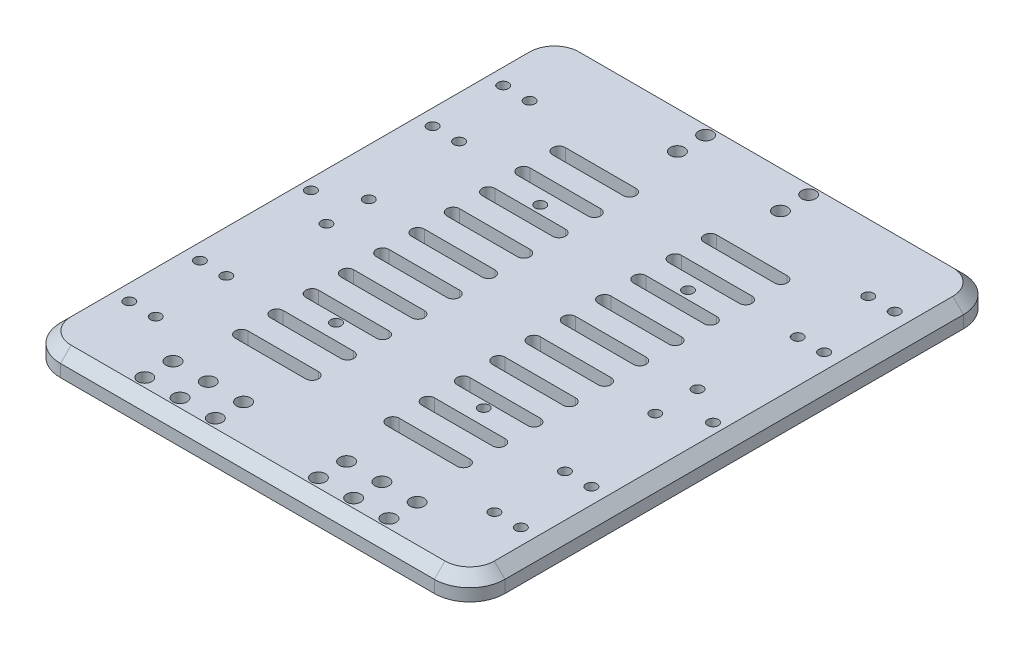
SolidWorks part; units mm, degrees
ref_plane "Front Plane" through (0, 0, 0) normal (0, 0, 1) x (1, 0, 0)
ref_plane "Top Plane" through (0, 0, 0) normal (0, 1, 0) x (1, 0, 0)
ref_plane "Right Plane" through (0, 0, 0) normal (1, 0, 0) x (0, 0, -1)
other "Configuration Table"
sketch "Sketch1" plane through (0, 0, 0) normal (0, 1, 0) x (1, 0, 0)
  line L1 (-63, -75) -> (63, -75)
  line L2 (-63, -75) -> (-63, 75)
  line L3 (-63, 75) -> (63, 75)
  line L4 (63, -75) -> (63, 75)
  line L5 (0, 75) -> (0, -75) construction
  line L6 (-63, 0) -> (63, 0) construction
  point P0 (0, 0)
  dimension "D1" = 126
  dimension "D2" = 150
extrude "Boss-Extrude1" add sketch "Sketch1" along normal blind 6.5
sketch "Sketch2" plane through (0, 6.5, 0) normal (0, 1, 0) x (1, 0, 0)
  line L0 (63, 75) -> (-63, 75) construction
  line L1 (-55.5, 33) -> (-48, 33) construction
  line L2 (-55.5, 33) -> (-55.5, 53) construction
  line L3 (-55.5, 53) -> (-48, 53) construction
  line L4 (-48, 33) -> (-48, 53) construction
  line L5 (-51.75, 53) -> (-51.75, 33) construction
  line L6 (-55.5, 43) -> (-48, 43) construction
  line L7 (-63, 75) -> (-63, -75) construction
  circle A0 centre (-55.5, 33) radius 1.5
  circle A1 centre (-48, 33) radius 1.5
  circle A2 centre (-48, 53) radius 1.5
  circle A3 centre (-55.5, 53) radius 1.5
  point P0 (-51.75, 43)
  dimension "D3" = 3
  dimension "D1" = 20
  dimension "D2" = 7.5
  dimension "D4" = 22
  dimension "D5" = 7.5
extrude "Cut-Extrude1" cut sketch "Sketch2" against normal blind 10
mirror "Mirror1" about plane through (0, 0, 0) normal (1, 0, 0) of "Cut-Extrude1"
mirror "Mirror2" about plane through (0, 0, 0) normal (0, 0, 1) of "Cut-Extrude1", "Mirror1"
fillet "Fillet1" radius 10 4 edges at (63, 3.25, 75) (-63, 3.25, 75) (63, 3.25, -75) (-63, 3.25, -75)
sketch "Sketch4" plane through (0, 6.5, 0) normal (0, 1, 0) x (1, 0, 0)
  line L0 (-63, 65) -> (-63, -65) construction
  line L1 (-57, 0) -> (-46.6077, -6) construction
  line L2 (-46.6077, -6) -> (-46.6077, 6) construction
  line L3 (-46.6077, 6) -> (-57, 0) construction
  circle A0 centre (-50.0718, 0) radius 3.4641 construction
  circle A1 centre (-46.6077, -6) radius 1.5
  circle A2 centre (-46.6077, 6) radius 1.5
  circle A3 centre (-57, 0) radius 1.5
  dimension "D3" = 3
  dimension "D1" = 12
  dimension "D2" = 6
extrude "Cut-Extrude3" cut sketch "Sketch4" against normal blind 10
mirror "Mirror3" about plane through (0, 0, 0) normal (1, 0, 0) of "Cut-Extrude3"
sketch "Sketch5" plane through (0, 6.5, 0) normal (0, 1, 0) x (1, 0, 0)
  line L0 (-53, -75) -> (53, -75) construction
  line L1 (63, -65) -> (63, 65) construction
  circle A0 centre (14.61, -61.5) radius 2
  circle A1 centre (14.61, -69.5) radius 2
  dimension "D1" = 4
  dimension "D2" = 13.5
  dimension "D3" = 48.39
  dimension "D4" = 8
extrude "Cut-Extrude4" cut sketch "Sketch5" against normal blind 20
mirror "Mirror4" about plane through (0, 0, 0) normal (1, 0, 0) of "Cut-Extrude4"
mirror "Mirror5" about plane through (0, 0, 0) normal (0, 0, 1) of "Cut-Extrude4", "Mirror4"
sketch "Sketch6" plane through (0, 6.5, 0) normal (0, 1, 0) x (1, 0, 0)
  circle A8 centre (14.61, -69.5) radius 2 construction
  circle A9 centre (14.61, -69.5) radius 2
  circle A10 centre (14.61, -61.5) radius 2 construction
  circle A11 centre (14.61, -61.5) radius 2
  circle A12 centre (24.61, -61.5) radius 2
  circle A13 centre (24.61, -69.5) radius 2
  circle A22 centre (34.61, -61.5) radius 2
  circle A23 centre (34.61, -69.5) radius 2
  circle A24 centre (-14.61, -61.5) radius 2 construction
  circle A25 centre (-14.61, -61.5) radius 2
  circle A26 centre (-14.61, -69.5) radius 2 construction
  circle A27 centre (-14.61, -69.5) radius 2
  circle A28 centre (-24.61, -61.5) radius 2
  circle A29 centre (-24.61, -69.5) radius 2
  circle A30 centre (-34.61, -61.5) radius 2
  circle A31 centre (-34.61, -69.5) radius 2
  dimension "D2" = 10
  dimension "D3" = 10
extrude "Cut-Extrude5" cut sketch "Sketch6" against normal through all
sketch "Sketch7" plane through (0, 6.5, 0) normal (0, 1, 0) x (1, 0, 0)
  line L0 (-31.4514, 44.7788) -> (-11.4514, 44.7788) construction
  line L1 (-31.4514, 46.5755) -> (-11.4514, 46.5755)
  line L2 (-31.4514, 42.9822) -> (-11.4514, 42.9822)
  line L3 (-31.4514, 34.7788) -> (-11.4514, 34.7788) construction
  line L4 (-31.4514, 36.5755) -> (-11.4514, 36.5755)
  line L5 (-31.4514, 32.9822) -> (-11.4514, 32.9822)
  line L6 (-31.4514, 24.7788) -> (-11.4514, 24.7788) construction
  line L7 (-31.4514, 26.5755) -> (-11.4514, 26.5755)
  line L8 (-31.4514, 22.9822) -> (-11.4514, 22.9822)
  line L9 (-31.4514, 14.7788) -> (-11.4514, 14.7788) construction
  line L10 (-31.4514, 16.5755) -> (-11.4514, 16.5755)
  line L11 (-31.4514, 12.9822) -> (-11.4514, 12.9822)
  line L12 (-31.4514, 4.7788) -> (-11.4514, 4.7788) construction
  line L13 (-31.4514, 6.5755) -> (-11.4514, 6.5755)
  line L14 (-31.4514, 2.9822) -> (-11.4514, 2.9822)
  line L15 (-31.4514, -5.2212) -> (-11.4514, -5.2212) construction
  line L16 (-31.4514, -3.4245) -> (-11.4514, -3.4245)
  line L17 (-31.4514, -7.0178) -> (-11.4514, -7.0178)
  line L18 (-31.4514, -15.2212) -> (-11.4514, -15.2212) construction
  line L19 (-31.4514, -13.4245) -> (-11.4514, -13.4245)
  line L20 (-31.4514, -17.0178) -> (-11.4514, -17.0178)
  line L21 (-31.4514, -25.2212) -> (-11.4514, -25.2212) construction
  line L22 (-31.4514, -23.4245) -> (-11.4514, -23.4245)
  line L23 (-31.4514, -27.0178) -> (-11.4514, -27.0178)
  line L24 (-31.4514, -35.2212) -> (-11.4514, -35.2212) construction
  line L25 (-31.4514, -33.4245) -> (-11.4514, -33.4245)
  line L26 (-31.4514, -37.0178) -> (-11.4514, -37.0178)
  line L27 (-31.4514, -45.2212) -> (-11.4514, -45.2212) construction
  line L28 (-31.4514, -43.4245) -> (-11.4514, -43.4245)
  line L29 (-31.4514, -47.0178) -> (-11.4514, -47.0178)
  line L30 (0, 0) -> (0, 32.0502) construction
  line L31 (31.4514, 44.7788) -> (11.4514, 44.7788) construction
  line L32 (31.4514, 46.5755) -> (11.4514, 46.5755)
  line L33 (31.4514, 42.9822) -> (11.4514, 42.9822)
  line L34 (31.4514, 34.7788) -> (11.4514, 34.7788) construction
  line L35 (31.4514, 36.5755) -> (11.4514, 36.5755)
  line L36 (31.4514, 32.9822) -> (11.4514, 32.9822)
  line L37 (31.4514, 24.7788) -> (11.4514, 24.7788) construction
  line L38 (31.4514, 26.5755) -> (11.4514, 26.5755)
  line L39 (31.4514, 22.9822) -> (11.4514, 22.9822)
  line L40 (31.4514, 14.7788) -> (11.4514, 14.7788) construction
  line L41 (31.4514, 16.5755) -> (11.4514, 16.5755)
  line L42 (31.4514, 12.9822) -> (11.4514, 12.9822)
  line L43 (31.4514, 4.7788) -> (11.4514, 4.7788) construction
  line L44 (31.4514, 6.5755) -> (11.4514, 6.5755)
  line L45 (31.4514, 2.9822) -> (11.4514, 2.9822)
  line L46 (31.4514, -5.2212) -> (11.4514, -5.2212) construction
  line L47 (31.4514, -3.4245) -> (11.4514, -3.4245)
  line L48 (31.4514, -7.0178) -> (11.4514, -7.0178)
  line L49 (31.4514, -15.2212) -> (11.4514, -15.2212) construction
  line L50 (31.4514, -13.4245) -> (11.4514, -13.4245)
  line L51 (31.4514, -17.0178) -> (11.4514, -17.0178)
  line L52 (31.4514, -25.2212) -> (11.4514, -25.2212) construction
  line L53 (31.4514, -23.4245) -> (11.4514, -23.4245)
  line L54 (31.4514, -27.0178) -> (11.4514, -27.0178)
  line L55 (31.4514, -35.2212) -> (11.4514, -35.2212) construction
  line L56 (31.4514, -33.4245) -> (11.4514, -33.4245)
  line L57 (31.4514, -37.0178) -> (11.4514, -37.0178)
  line L58 (31.4514, -45.2212) -> (11.4514, -45.2212) construction
  line L59 (31.4514, -43.4245) -> (11.4514, -43.4245)
  line L60 (31.4514, -47.0178) -> (11.4514, -47.0178)
  arc A0 (-31.4514, 46.5755) -> (-31.4514, 42.9822) centre (-31.4514, 44.7788) ccw
  arc A1 (-11.4514, 42.9822) -> (-11.4514, 46.5755) centre (-11.4514, 44.7788) ccw
  arc A2 (-31.4514, 36.5755) -> (-31.4514, 32.9822) centre (-31.4514, 34.7788) ccw
  arc A3 (-11.4514, 32.9822) -> (-11.4514, 36.5755) centre (-11.4514, 34.7788) ccw
  arc A4 (-31.4514, 26.5755) -> (-31.4514, 22.9822) centre (-31.4514, 24.7788) ccw
  arc A5 (-11.4514, 22.9822) -> (-11.4514, 26.5755) centre (-11.4514, 24.7788) ccw
  arc A6 (-31.4514, 16.5755) -> (-31.4514, 12.9822) centre (-31.4514, 14.7788) ccw
  arc A7 (-11.4514, 12.9822) -> (-11.4514, 16.5755) centre (-11.4514, 14.7788) ccw
  arc A8 (-31.4514, 6.5755) -> (-31.4514, 2.9822) centre (-31.4514, 4.7788) ccw
  arc A9 (-11.4514, 2.9822) -> (-11.4514, 6.5755) centre (-11.4514, 4.7788) ccw
  arc A10 (-31.4514, -3.4245) -> (-31.4514, -7.0178) centre (-31.4514, -5.2212) ccw
  arc A11 (-11.4514, -7.0178) -> (-11.4514, -3.4245) centre (-11.4514, -5.2212) ccw
  arc A12 (-31.4514, -13.4245) -> (-31.4514, -17.0178) centre (-31.4514, -15.2212) ccw
  arc A13 (-11.4514, -17.0178) -> (-11.4514, -13.4245) centre (-11.4514, -15.2212) ccw
  arc A14 (-31.4514, -23.4245) -> (-31.4514, -27.0178) centre (-31.4514, -25.2212) ccw
  arc A15 (-11.4514, -27.0178) -> (-11.4514, -23.4245) centre (-11.4514, -25.2212) ccw
  arc A16 (-31.4514, -33.4245) -> (-31.4514, -37.0178) centre (-31.4514, -35.2212) ccw
  arc A17 (-11.4514, -37.0178) -> (-11.4514, -33.4245) centre (-11.4514, -35.2212) ccw
  arc A18 (-31.4514, -43.4245) -> (-31.4514, -47.0178) centre (-31.4514, -45.2212) ccw
  arc A19 (-11.4514, -47.0178) -> (-11.4514, -43.4245) centre (-11.4514, -45.2212) ccw
  arc A20 (31.4514, 46.5755) -> (31.4514, 42.9822) centre (31.4514, 44.7788) cw
  arc A21 (11.4514, 42.9822) -> (11.4514, 46.5755) centre (11.4514, 44.7788) cw
  arc A22 (31.4514, 36.5755) -> (31.4514, 32.9822) centre (31.4514, 34.7788) cw
  arc A23 (11.4514, 32.9822) -> (11.4514, 36.5755) centre (11.4514, 34.7788) cw
  arc A24 (31.4514, 26.5755) -> (31.4514, 22.9822) centre (31.4514, 24.7788) cw
  arc A25 (11.4514, 22.9822) -> (11.4514, 26.5755) centre (11.4514, 24.7788) cw
  arc A26 (31.4514, 16.5755) -> (31.4514, 12.9822) centre (31.4514, 14.7788) cw
  arc A27 (11.4514, 12.9822) -> (11.4514, 16.5755) centre (11.4514, 14.7788) cw
  arc A28 (31.4514, 6.5755) -> (31.4514, 2.9822) centre (31.4514, 4.7788) cw
  arc A29 (11.4514, 2.9822) -> (11.4514, 6.5755) centre (11.4514, 4.7788) cw
  arc A30 (31.4514, -3.4245) -> (31.4514, -7.0178) centre (31.4514, -5.2212) cw
  arc A31 (11.4514, -7.0178) -> (11.4514, -3.4245) centre (11.4514, -5.2212) cw
  arc A32 (31.4514, -13.4245) -> (31.4514, -17.0178) centre (31.4514, -15.2212) cw
  arc A33 (11.4514, -17.0178) -> (11.4514, -13.4245) centre (11.4514, -15.2212) cw
  arc A34 (31.4514, -23.4245) -> (31.4514, -27.0178) centre (31.4514, -25.2212) cw
  arc A35 (11.4514, -27.0178) -> (11.4514, -23.4245) centre (11.4514, -25.2212) cw
  arc A36 (31.4514, -33.4245) -> (31.4514, -37.0178) centre (31.4514, -35.2212) cw
  arc A37 (11.4514, -37.0178) -> (11.4514, -33.4245) centre (11.4514, -35.2212) cw
  arc A38 (31.4514, -43.4245) -> (31.4514, -47.0178) centre (31.4514, -45.2212) cw
  arc A39 (11.4514, -47.0178) -> (11.4514, -43.4245) centre (11.4514, -45.2212) cw
  point P2 (-21.4514, 44.7788)
  point P10 (-21.4514, 34.7788)
  point P17 (-21.4514, 24.7788)
  point P24 (-21.4514, 14.7788)
  point P31 (-21.4514, 4.7788)
  point P38 (-21.4514, -5.2212)
  point P45 (-21.4514, -15.2212)
  point P52 (-21.4514, -25.2212)
  point P59 (-21.4514, -35.2212)
  point P66 (-21.4514, -45.2212)
  point P75 (21.4514, 44.7788)
  point P82 (21.4514, 34.7788)
  point P89 (21.4514, 24.7788)
  point P96 (21.4514, 14.7788)
  point P103 (21.4514, 4.7788)
  point P110 (21.4514, -5.2212)
  point P117 (21.4514, -15.2212)
  point P124 (21.4514, -25.2212)
  point P131 (21.4514, -35.2212)
  point P138 (21.4514, -45.2212)
  dimension "D1" = 20
  dimension "D2" = 10
extrude "Cut-Extrude6" cut sketch "Sketch7" against normal through all
chamfer "Chamfer1" distance 3 angle 45 8 edges at (-63, 6.5, 0) (-60.0711, 6.5, 72.0711) (-60.0711, 6.5, -72.0711) (0, 6.5, 75) (0, 6.5, -75) (60.0711, 6.5, 72.0711) (60.0711, 6.5, -72.0711) (63, 6.5, 0)
sketch "Sketch8" plane through (0, 0, 0) normal (0, -1, 0) x (1, 0, 0)
  line L1 (-20.95, -28.95) -> (20.95, -28.95) construction
  line L2 (-20.95, -28.95) -> (-20.95, 28.95) construction
  line L3 (-20.95, 28.95) -> (20.95, 28.95) construction
  line L4 (20.95, -28.95) -> (20.95, 28.95) construction
  line L5 (0, 28.95) -> (0, -28.95) construction
  line L6 (-20.95, 0) -> (20.95, 0) construction
  circle A1 centre (20.95, -28.95) radius 1.5
  circle A2 centre (-20.95, -28.95) radius 1.5
  circle A3 centre (20.95, 28.95) radius 1.5
  circle A4 centre (-20.95, 28.95) radius 1.5
  point P0 (0, 0)
  dimension "D3" = 3
  dimension "D1" = 41.9
  dimension "D2" = 57.9
extrude "Cut-Extrude7" cut sketch "Sketch8" against normal through all
